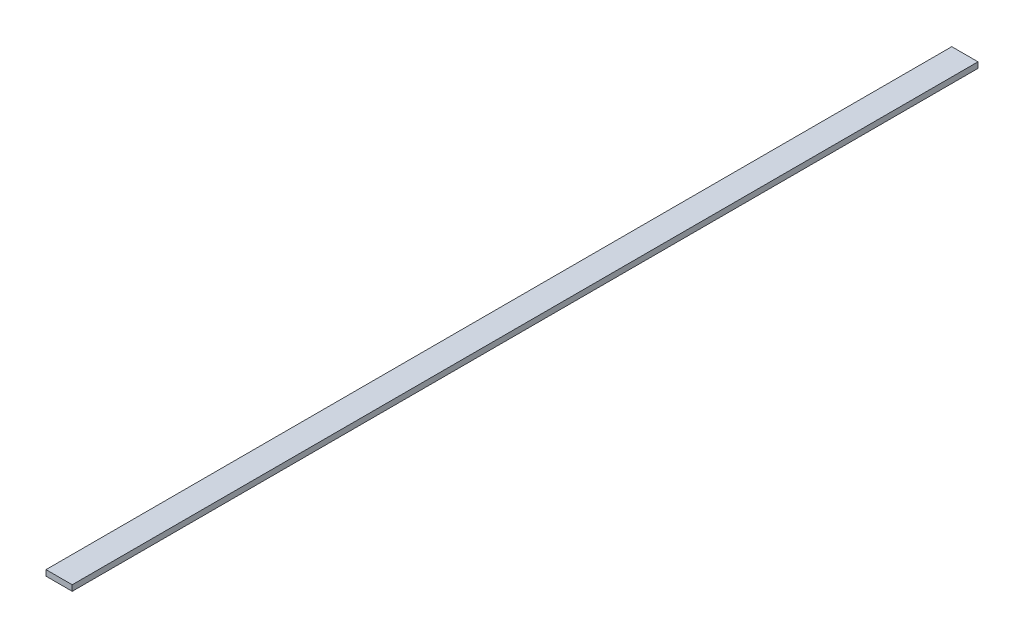
SolidWorks part; units mm, degrees
ref_plane "前视基准面" through (0, 0, 0) normal (0, 0, 1) x (1, 0, 0)
ref_plane "上视基准面" through (0, 0, 0) normal (0, 1, 0) x (1, 0, 0)
ref_plane "右视基准面" through (0, 0, 0) normal (1, 0, 0) x (0, 0, -1)
other "Configuration Table"
sketch "草图1" plane through (0, 0, 0) normal (0, 0, 1) x (1, 0, 0)
  line L1 (0, 0) -> (55, 0)
  line L2 (0, 0) -> (0, -12)
  line L3 (0, -12) -> (55, -12)
  line L4 (55, 0) -> (55, -12)
  dimension "D1" = 55
  dimension "D2" = 12
extrude "凸台-拉伸1" add sketch "草图1" along normal blind 1900
